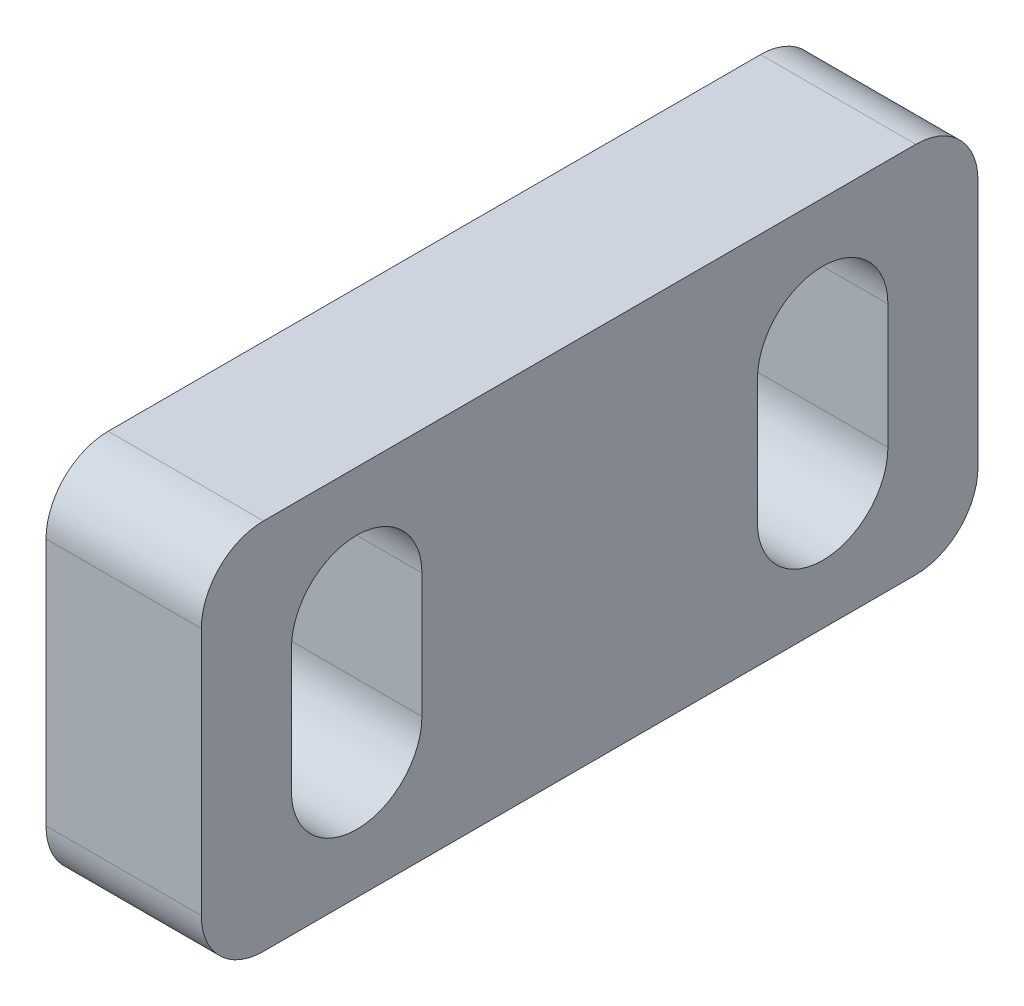
SolidWorks part; units mm, degrees
material "A3钢"
ref_plane "前视基准面" through (0, 0, 0) normal (0, 0, 1) x (1, 0, 0)
ref_plane "上视基准面" through (0, 0, 0) normal (0, 1, 0) x (1, 0, 0)
ref_plane "右视基准面" through (0, 0, 0) normal (1, 0, 0) x (0, 0, -1)
sketch "草图1" plane through (0, 0, 0) normal (1, 0, 0) x (0, 0, -1)
  line L0 (0, 33.5) -> (0, -7.9603) construction
  line L1 (-12.5, 6) -> (-6, 6)
  line L2 (-12.5, 6) -> (-12.5, -6)
  line L3 (-12.5, -6) -> (12.5, -6)
  line L4 (12.5, 6) -> (12.5, -6)
  line L5 (-12.5, 6) -> (12.5, -6) construction
  line L6 (-12.5, -6) -> (12.5, 6) construction
  line L7 (-6, 61) -> (6, 61)
  line L8 (-6, 61) -> (-6, 6)
  line L10 (6, 61) -> (6, 6)
  line L11 (-6, 61) -> (6, 6) construction
  line L12 (-6, 6) -> (6, 61) construction
  line L14 (6, 6) -> (12.5, 6)
  point P0 (0, 0)
  point P6 (0, 33.5)
  dimension "D1" = 12
  dimension "D2" = 25
  dimension "D3" = 12
  dimension "D4" = 55
extrude "凸台-拉伸1" add sketch "草图1" along normal blind 5
sketch "草图2" plane through (0, 0, 0) normal (-1, 0, 0) x (0, 0, 1)
  line L0 (-6, 61) -> (-12.5, 6)
  line L1 (6, 61) -> (12.5, 6)
  line L2 (-6, 61) -> (6, 61)
  line L3 (-12.5, 6) -> (12.5, 6)
extrude "凸台-拉伸2" add sketch "草图2" against normal up to surface (5 mm away) up to face at (5, 16.75, 0)
fillet "圆角1" radius 2 2 edges at (2.5, 61, 6) (2.5, 61, -6)
sketch "草图3" plane through (0, 0, 0) normal (-1, 0, 0) x (0, 0, 1)
  line L0 (-9.6408, 0) -> (9.298, 0) construction
  line L1 (0, 0) -> (0, -6.9973) construction
  line L2 (-7.5, 2) -> (-7.5, -2) construction
  line L3 (-5.4, 2) -> (-5.4, -2)
  line L4 (-9.6, 2) -> (-9.6, -2)
  line L5 (7.5, 2) -> (7.5, -2) construction
  line L6 (5.4, 2) -> (5.4, -2)
  line L7 (9.6, 2) -> (9.6, -2)
  line L8 (12.5, -6) -> (-12.5, -6) construction
  arc A0 (-5.4, 2) -> (-9.6, 2) centre (-7.5, 2) ccw
  arc A1 (-9.6, -2) -> (-5.4, -2) centre (-7.5, -2) ccw
  arc A2 (5.4, 2) -> (9.6, 2) centre (7.5, 2) cw
  arc A3 (9.6, -2) -> (5.4, -2) centre (7.5, -2) cw
  point P7 (-7.5, 0)
  point P14 (7.5, 0)
  dimension "D4" = 2.1
  dimension "D1" = 15
  dimension "D2" = 4
  dimension "D3" = 6
extrude "切除-拉伸1" cut sketch "草图3" against normal blind 13
fillet "圆角2" radius 2 2 edges at (2.5, -6, -12.5) (2.5, -6, 12.5)
hole_wizard "Ø4.3 (4.3) 直径孔1" positions "草图4" profile "草图6" hole size "Ø4.3" standard "GB"
sketch "草图4" plane through (0, 0, 0) normal (-1, 0, 0) x (0, 0, 1)
  point P0 (0, 56)
  point P3 (0, 41)
sketch "草图6" plane through (0, 56, 0) normal (0, 1, 0) x (0, 0, 1)
  line L0 (0, 0) -> (0, 11.3919)
  line L1 (0, 11.3919) -> (2.15, 10.1)
  line L2 (2.15, 10.1) -> (2.15, 0)
  line L5 (2.15, 0) -> (0, 0)
  line L10 (0, 11.3919) -> (-2.15, 10.1) construction
  line L11 (0, -6.35) -> (0, 107.95) construction
  dimension "孔直径" = 4.3
  dimension "孔深度" = 10.1
  dimension "导头角度" = 118
sketch "草图7" plane through (5, 0, 0) normal (1, 0, 0) x (0, 0, -1)
  line L0 (4.2224, 61) -> (-4.2224, 61) construction
  line L1 (-13.476, 63.8853) -> (10.9733, 63.8853)
  line L2 (-13.476, 63.8853) -> (-13.476, 36)
  line L3 (-13.476, 36) -> (10.9733, 36)
  line L4 (10.9733, 63.8853) -> (10.9733, 36)
  dimension "D1" = 25
extrude "切除-拉伸2" cut sketch "草图7" against normal blind 10
sketch "草图8" plane through (0, 0, 0) normal (-1, 0, 0) x (0, 0, 1)
  line L0 (-1, 31.5) -> (1, 31.5) construction
  line L1 (-1, 33.75) -> (1, 33.75)
  line L2 (-1, 29.25) -> (1, 29.25)
  line L3 (8.9545, 36) -> (-8.9545, 36) construction
  line L4 (0, 0) -> (0, 48.2057) construction
  arc A0 (-1, 33.75) -> (-1, 29.25) centre (-1, 31.5) ccw
  arc A1 (1, 29.25) -> (1, 33.75) centre (1, 31.5) ccw
  point P2 (0, 31.5)
  dimension "D1" = 2.25
  dimension "D2" = 4.5
  dimension "D3" = 2
extrude "切除-拉伸3" cut sketch "草图8" against normal blind 10
fillet "圆角3" radius 5 2 edges at (2.5, 36, -8.9545) (2.5, 36, 8.9545)
sketch "草图9" plane through (5, 0, 0) normal (1, 0, 0) x (0, 0, -1)
  line L0 (-10.5, -6) -> (10.5, -6) construction
  line L1 (15.3918, 6) -> (-21.4048, 6)
  line L2 (15.3918, 6) -> (15.3918, 38.1562)
  line L3 (15.3918, 38.1562) -> (-21.4048, 38.1562)
  line L4 (-21.4048, 6) -> (-21.4048, 38.1562)
  dimension "D1" = 12
extrude "切除-拉伸4" cut sketch "草图9" against normal blind 21
fillet "圆角4" radius 2 2 edges at (2.5, 6, 12.5) (2.5, 6, -12.5)
